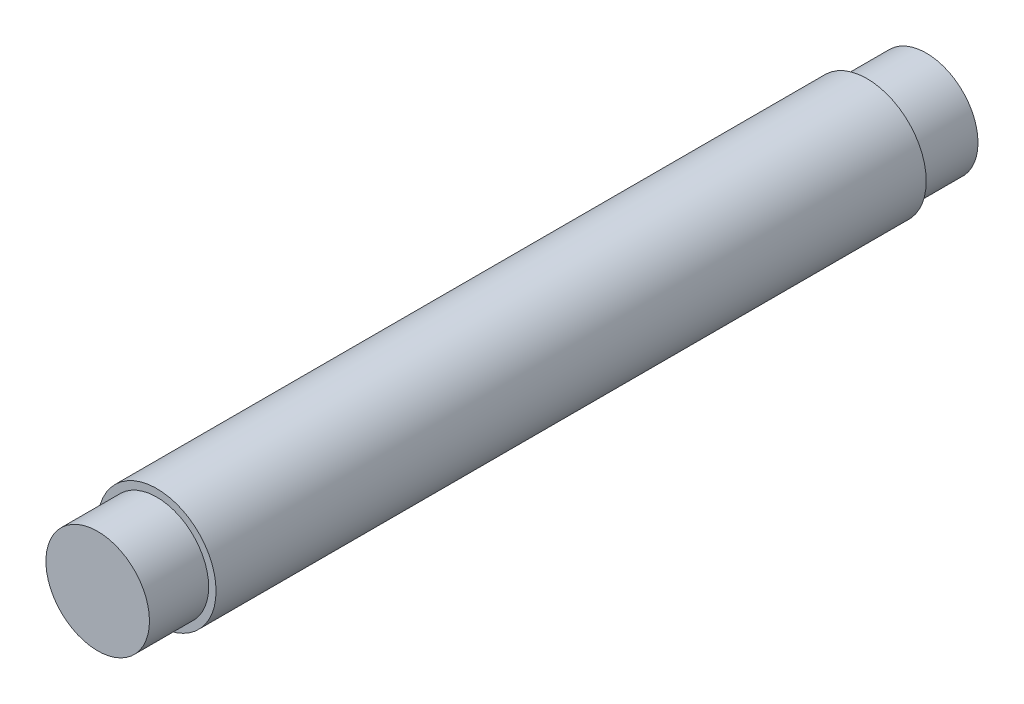
SolidWorks part; units mm, degrees
ref_plane "Front Plane" through (0, 0, 0) normal (0, 0, 1) x (1, 0, 0)
ref_plane "Top Plane" through (0, 0, 0) normal (0, 1, 0) x (1, 0, 0)
ref_plane "Right Plane" through (0, 0, 0) normal (1, 0, 0) x (0, 0, -1)
other "Configuration Table"
sketch "Sketch1" plane through (0, 0, 0) normal (0, 0, 1) x (1, 0, 0)
  circle A0 centre (0, 0) radius 87.5
  dimension "D1" = 175
extrude "Boss-Extrude1" add sketch "Sketch1" along normal mid plane 1400
sketch "Sketch2" plane through (0, 0, 0) normal (0, 0, 1) x (1, 0, 0)
  circle A0 centre (0, 0) radius 100
  dimension "D1" = 200
extrude "Boss-Extrude2" add sketch "Sketch2" along normal mid plane 1200
